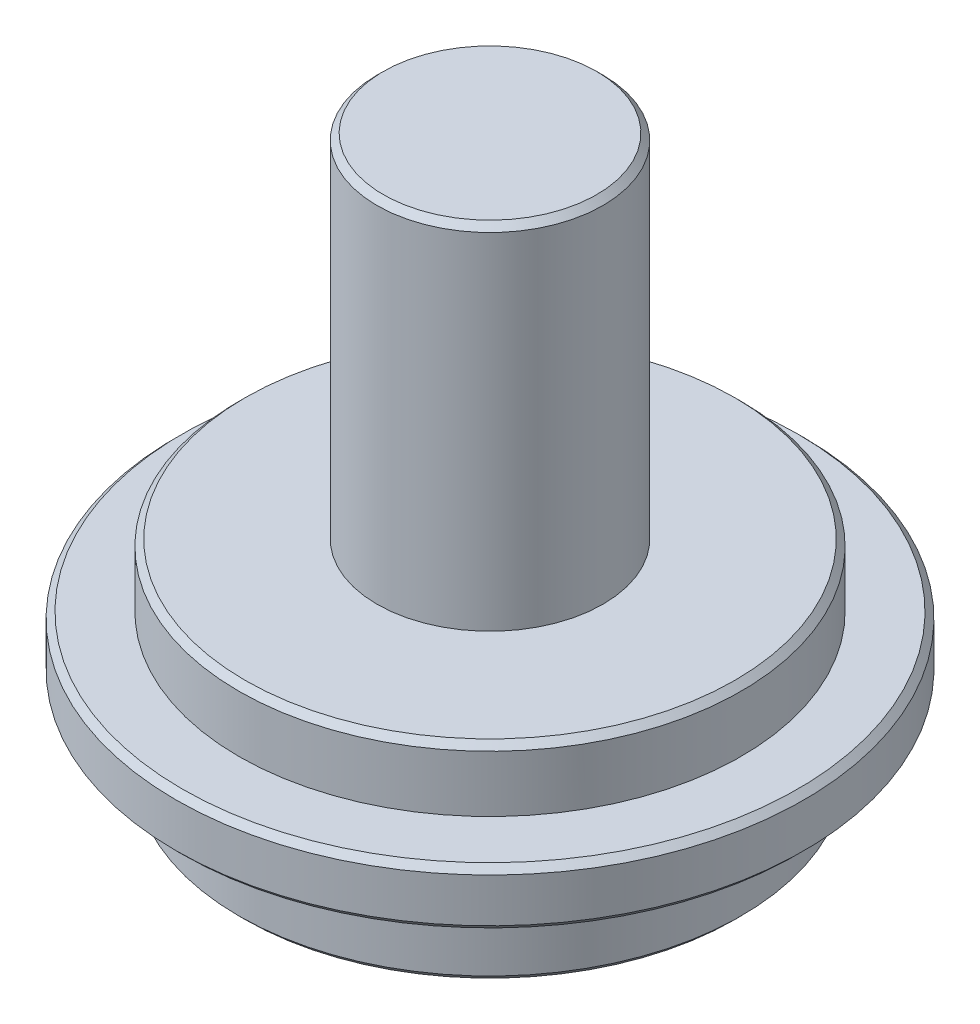
from build123d import *

# Parameters (mm, degrees)
CHAMFER1_SIZE = 0.5


with BuildPart() as part:
    # Sketch1 → Revolve1 (revolve)
    with BuildSketch(Plane.XY, mode=Mode.PRIVATE) as revolve1_sk:
        Polygon((258.314300847, -567), (258.314300847, -595), (269.314300847, -595), (269.314300847, -600), (274.314300847, -600), (274.314300847, -604.5), (269.314300847, -604.5), (269.314300847, -611.5), (249.314300847, -611.5), (249.314300847, -567), align=None)
    revolve(revolve1_sk.sketch.rotate(Axis((249.314300847, -567, 0), (0, -1, 0)), 90), axis=Axis((249.314300847, -567, 0), (0, -1, 0)))

    # Chamfer1
    chamfer1_edges = [part.edges().sort_by_distance(p)[0] for p in [
        (249.314300847, -604.5, -25),
        (249.314300847, -611.5, -20),
        (249.314300847, -567, -9),
        (249.314300847, -595, -20),
        (249.314300847, -600, -25),
    ]]
    chamfer(chamfer1_edges, length=CHAMFER1_SIZE)


solid = part.part
